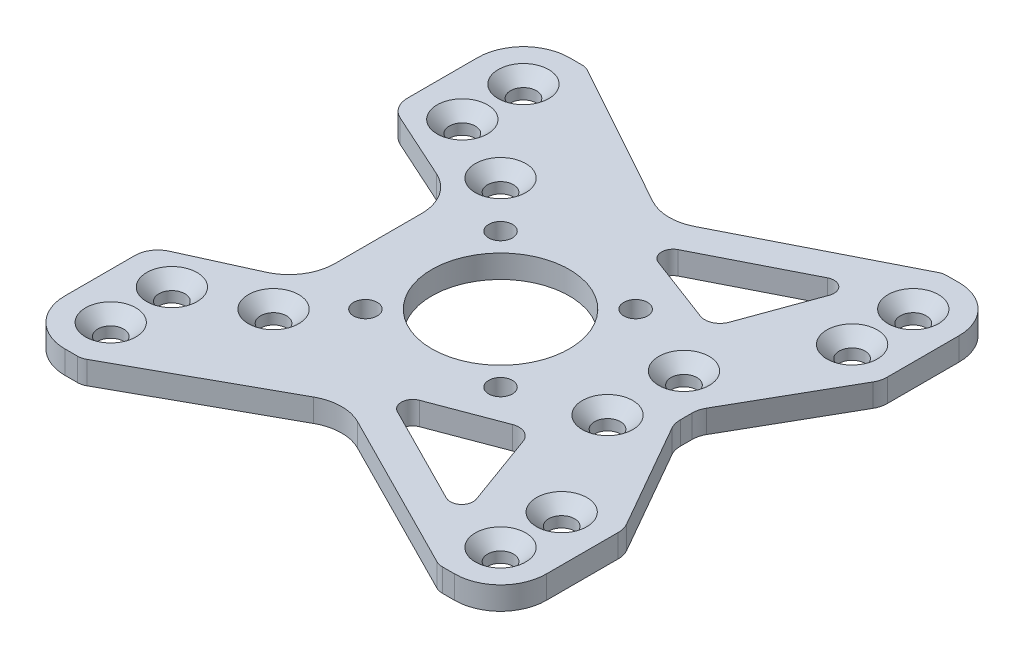
from build123d import *

# Parameters (mm, degrees)
SKETCH_1_W                   = 66
SKETCH_1_H                   = 66
SKETCH_1_R                   = 9
SKETCH_1_R_2                 = 1.55
EXTRUDE_1_DEPTH              = 3
HOLE_WIZARD_M3_1_D           = 3.4
HOLE_WIZARD_M3_1_DEPTH       = 7.5
HOLE_WIZARD_M3_1_CSINK_D     = 6.6
HOLE_WIZARD_M3_1_CSINK_ANGLE = 90
HOLE_WIZARD_M3_1_TIP         = 1.021463052
CUT_EXTRUDE_3_DEPTH          = 47.765371804
CUT_EXTRUDE_3_DEPTH_BACK     = 47.765371804
SKETCH_8_W                   = 3
SKETCH_8_H                   = 66
FILLET_1_R                   = 6
CUT_EXTRUDE_2_DEPTH          = 47.765371804
FILLET_2_R                   = 2
FILLET_3_R                   = 1.5
FILLET_4_R                   = 6
FILLET_5_R                   = 3


with BuildPart() as part:
    # 草图1 → 凸台-拉伸1 (new body)
    with BuildSketch(Plane(origin=(0, 0, 0), x_dir=(1, 0, 0), z_dir=(0, 1, 0))):
        Rectangle(SKETCH_1_W, SKETCH_1_H)
        with Locations(Location((0, 0, 0), (0, 0, 270))):
            Circle(SKETCH_1_R, mode=Mode.SUBTRACT)
        with Locations(Location((-24, 19, 0), (0, 0, 270))):
            Circle(SKETCH_1_R_2, mode=Mode.SUBTRACT)
        with Locations(Location((-24, 27, 0), (0, 0, 270))):
            Circle(SKETCH_1_R_2, mode=Mode.SUBTRACT)
        with Locations(Location((-24, -19, 0), (0, 0, 90))):
            Circle(SKETCH_1_R_2, mode=Mode.SUBTRACT)
        with Locations(Location((-24, -27, 0), (0, 0, 90))):
            Circle(SKETCH_1_R_2, mode=Mode.SUBTRACT)
        with Locations(Location((-14.849242405, 14.849242405, 0), (0, 0, 270))):
            Circle(SKETCH_1_R_2, mode=Mode.SUBTRACT)
        with Locations(Location((19, 5, 0), (0, 0, 270))):
            Circle(SKETCH_1_R_2, mode=Mode.SUBTRACT)
        with Locations(Location((19, -5, 0), (0, 0, 90))):
            Circle(SKETCH_1_R_2, mode=Mode.SUBTRACT)
        with Locations(Location((-14.849242405, -14.849242405, 0), (0, 0, 90))):
            Circle(SKETCH_1_R_2, mode=Mode.SUBTRACT)
        with Locations(Location((8.838834765, 8.838834765, 0), (0, 0, 270))):
            Circle(SKETCH_1_R_2, mode=Mode.SUBTRACT)
        with Locations(Location((8.838834765, -8.838834765, 0), (0, 0, 270))):
            Circle(SKETCH_1_R_2, mode=Mode.SUBTRACT)
        with Locations(Location((-8.838834765, -8.838834765, 0), (0, 0, 270))):
            Circle(SKETCH_1_R_2, mode=Mode.SUBTRACT)
        with Locations(Location((-8.838834765, 8.838834765, 0), (0, 0, 270))):
            Circle(SKETCH_1_R_2, mode=Mode.SUBTRACT)
        with Locations(Location((27, 27, 0), (0, 0, 270))):
            Circle(SKETCH_1_R_2, mode=Mode.SUBTRACT)
        with Locations(Location((27, 19, 0), (0, 0, 270))):
            Circle(SKETCH_1_R_2, mode=Mode.SUBTRACT)
        with Locations(Location((27, -19, 0), (0, 0, 90))):
            Circle(SKETCH_1_R_2, mode=Mode.SUBTRACT)
        with Locations(Location((27, -27, 0), (0, 0, 90))):
            Circle(SKETCH_1_R_2, mode=Mode.SUBTRACT)
    extrude(amount=EXTRUDE_1_DEPTH)

    # M3 十字槽半沉头木螺钉的锥形沉头孔1
    with Locations(Plane(origin=(0, 3, 0), x_dir=(1, 0, 0), z_dir=(0, 1, 0))):
        with Locations((-24, 27), (-24, 19), (-24, -19), (-24, -27), (-14.849242405, 14.849242405), (-14.849242405, -14.849242405), (19, -5), (19, 5), (27, 19), (27, 27), (27, -19), (27, -27)):
            CounterSinkHole(HOLE_WIZARD_M3_1_D / 2, HOLE_WIZARD_M3_1_CSINK_D / 2, depth=HOLE_WIZARD_M3_1_DEPTH, counter_sink_angle=HOLE_WIZARD_M3_1_CSINK_ANGLE)
            with Locations((0, 0, -(HOLE_WIZARD_M3_1_DEPTH + HOLE_WIZARD_M3_1_TIP / 2))):  # 118° drill point
                Cone(0, HOLE_WIZARD_M3_1_D / 2, HOLE_WIZARD_M3_1_TIP, mode=Mode.SUBTRACT)

    # 草图8 → 切除-拉伸3 (cut, two sides: drawn at the far end of the back side and taken through both)
    with BuildSketch(Plane(origin=(0, 3, 0), x_dir=(1, 0, 0), z_dir=(0, 1, 0)).offset(-CUT_EXTRUDE_3_DEPTH_BACK)):
        with Locations((-31.5, 0)):
            Rectangle(SKETCH_8_W, SKETCH_8_H)
    extrude(amount=CUT_EXTRUDE_3_DEPTH + CUT_EXTRUDE_3_DEPTH_BACK, mode=Mode.SUBTRACT)

    # 圆角1
    fillet_1_edges = [part.edges().sort_by_distance(p)[0] for p in [
        (-30, 1.5, -33),
        (-30, 1.5, 33),
        (33, 1.5, 33),
        (33, 1.5, -33),
    ]]
    fillet(fillet_1_edges, radius=FILLET_1_R)

    # 草图5 → 切除-拉伸2 (cut, through all)
    with BuildSketch(Plane(origin=(0, 3, 0), x_dir=(1, 0, 0), z_dir=(0, 1, 0))):
        Polygon((-31, 16.355426805), (-31, -16.355426805), (-16, -9.551469506), (-16, 9.551469506), align=None)
        Polygon((34, 18.551944046), (24.3, 1.576944046), (24.3, -1.576944046), (34, -18.551944046), align=None)
        Polygon((-23.639707799, 34), (26.876227293, 34), (0.514933103, 20.641535007), align=None)
        Polygon((21.235931274, 26.657538386), (1.839031633, 16.828248406), (15.750489279, 11.5725729), align=None)
        Polygon((1.839031633, -16.828248406), (15.750489279, -11.5725729), (21.235931274, -26.657538386), align=None)
        Polygon((26.876227293, -34), (0.514933103, -20.641535007), (-23.639707799, -34), align=None)
    extrude(amount=-CUT_EXTRUDE_2_DEPTH, mode=Mode.SUBTRACT)

    # 圆角2
    fillet_2_edges = [part.edges().sort_by_distance(p)[0] for p in [
        (24.902849797, 1.5, 33),
        (-21.831517943, 1.5, 33),
        (-21.831517943, 1.5, -33),
        (24.902849797, 1.5, -33),
        (15.750489279, 1.5, 11.5725729),
        (15.750489279, 1.5, -11.5725729),
    ]]
    fillet(fillet_2_edges, radius=FILLET_2_R)

    # 圆角3
    fillet_3_edges = [part.edges().sort_by_distance(p)[0] for p in [
        (21.235931274, 1.5, 26.657538386),
        (1.839031633, 1.5, 16.828248406),
        (21.235931274, 1.5, -26.657538386),
        (1.839031633, 1.5, -16.828248406),
    ]]
    fillet(fillet_3_edges, radius=FILLET_3_R)

    # 圆角4
    fillet_4_edges = [part.edges().sort_by_distance(p)[0] for p in [
        (0.514933103, 1.5, -20.641535007),
        (0.514933103, 1.5, 20.641535007),
        (-16, 1.5, 9.551469506),
        (-16, 1.5, -9.551469506),
    ]]
    fillet(fillet_4_edges, radius=FILLET_4_R)

    # 圆角5
    fillet_5_edges = [part.edges().sort_by_distance(p)[0] for p in [
        (-30, 1.5, -15.901829651),
        (-30, 1.5, 15.901829651),
        (33, 1.5, 16.801944046),
        (33, 1.5, -16.801944046),
        (24.3, 1.5, -1.576944046),
        (24.3, 1.5, 1.576944046),
    ]]
    fillet(fillet_5_edges, radius=FILLET_5_R)


solid = part.part
